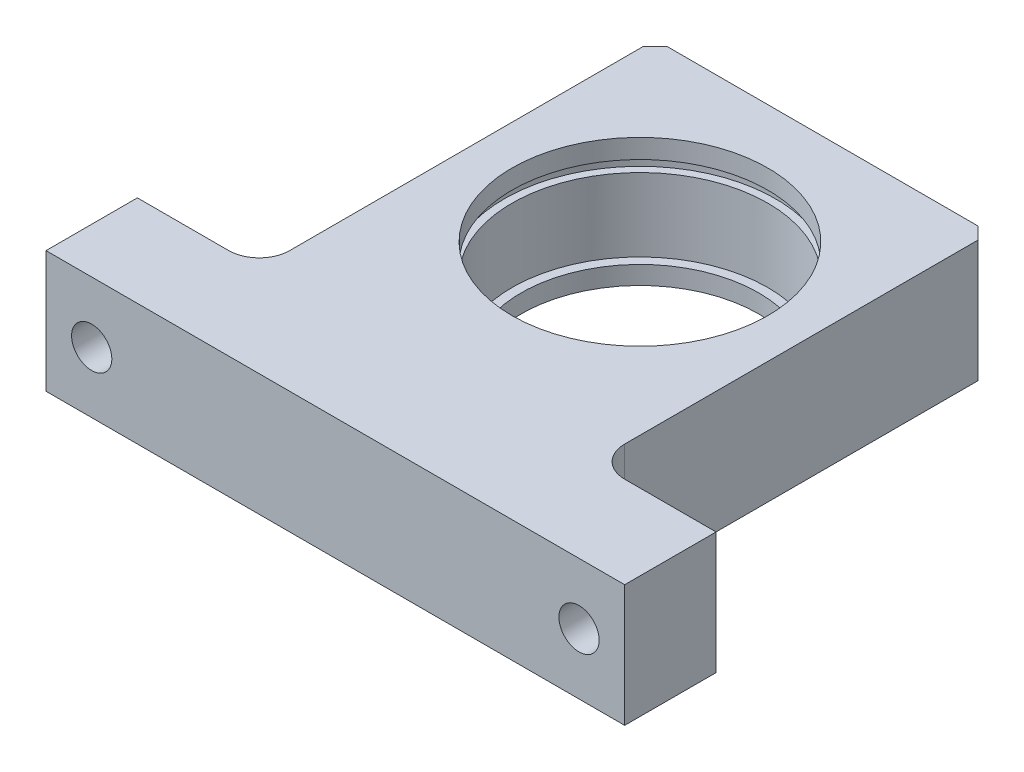
SolidWorks part; units mm, degrees
ref_plane "前视基准面" through (0, 0, 0) normal (0, 0, 1) x (1, 0, 0)
ref_plane "上视基准面" through (0, 0, 0) normal (0, 1, 0) x (1, 0, 0)
ref_plane "右视基准面" through (0, 0, 0) normal (1, 0, 0) x (0, 0, -1)
sketch "草图1" plane through (0, 0, 0) normal (0, 1, 0) x (1, 0, 0)
  line L0 (-47.5, 0) -> (47.5, 0)
  line L1 (-47.5, 0) -> (-47.5, 15)
  line L2 (-47.5, 15) -> (-27.5, 15)
  line L3 (-27.5, 15) -> (-27.5, 80)
  line L4 (-27.5, 80) -> (27.5, 80)
  line L5 (27.5, 80) -> (27.5, 15)
  line L6 (27.5, 15) -> (47.5, 15)
  line L7 (47.5, 15) -> (47.5, 0)
  line L8 (0, 0) -> (0, 147.7709) construction
  circle A0 centre (0, 50) radius 21
  point P4 (0, 0)
  dimension "D1" = 42
  dimension "D2" = 80
  dimension "D3" = 30
  dimension "D4" = 55
  dimension "D5" = 20
  dimension "D6" = 15
extrude "凸台-拉伸1" add sketch "草图1" along normal blind 20
chamfer "倒角1" distance 2 angle 45 2 edges at (27.5, 10, -80) (-27.5, 10, -80)
fillet "圆角1" radius 5 2 edges at (27.5, 10, -15) (-27.5, 10, -15)
sketch "草图2" plane through (0, 0, 0) normal (0, -1, 0) x (1, 0, 0)
  circle A0 centre (0, -50) radius 21 construction
  circle A1 centre (0, -50) radius 21
  circle A2 centre (0, -50) radius 19.5
  dimension "D1" = 1.5
extrude "凸台-拉伸2" add sketch "草图2" against normal blind 3
sketch "草图8" plane through (0, 0, -15) normal (0, 0, -1) x (-1, 0, 0)
  line L0 (0, 0) -> (0, 27.0331) construction
  line L2 (-47.5, 20) -> (-47.5, 0) construction
  point P0 (-40, 10)
  point P7 (40, 10)
  point P10 (-47.5, 10)
  dimension "D1" = 80
hole_wizard "M6 间隙孔1" positions "草图8" profile "草图7" hole size "M6" standard "GB" end condition through all
sketch "草图7" plane through (40, 10, -15) normal (1, 0, 0) x (0, 1, 0)
  line L0 (0, 0) -> (0, 15)
  line L1 (0, 15) -> (3.3, 15)
  line L2 (3.3, 15) -> (3.3, 0)
  line L5 (3.3, 0) -> (0, 0)
  line L11 (0, -6.35) -> (0, 107.95) construction
  dimension "通孔孔直径" = 6.6
  dimension "通孔孔深度" = 15
ref_plane "基准面1" through (0, 15, 0) normal (0, 1, 0) x (1, 0, 0)
sketch "草图9" plane through (0, 15, 0) normal (0, 1, 0) x (1, 0, 0)
  circle A0 centre (0, 50) radius 21 construction
  circle A1 centre (0, 50) radius 21
  circle A2 centre (0, 50) radius 22.25
  dimension "D1" = 44.5
extrude "切除-拉伸1" cut sketch "草图9" along normal blind 1.85
